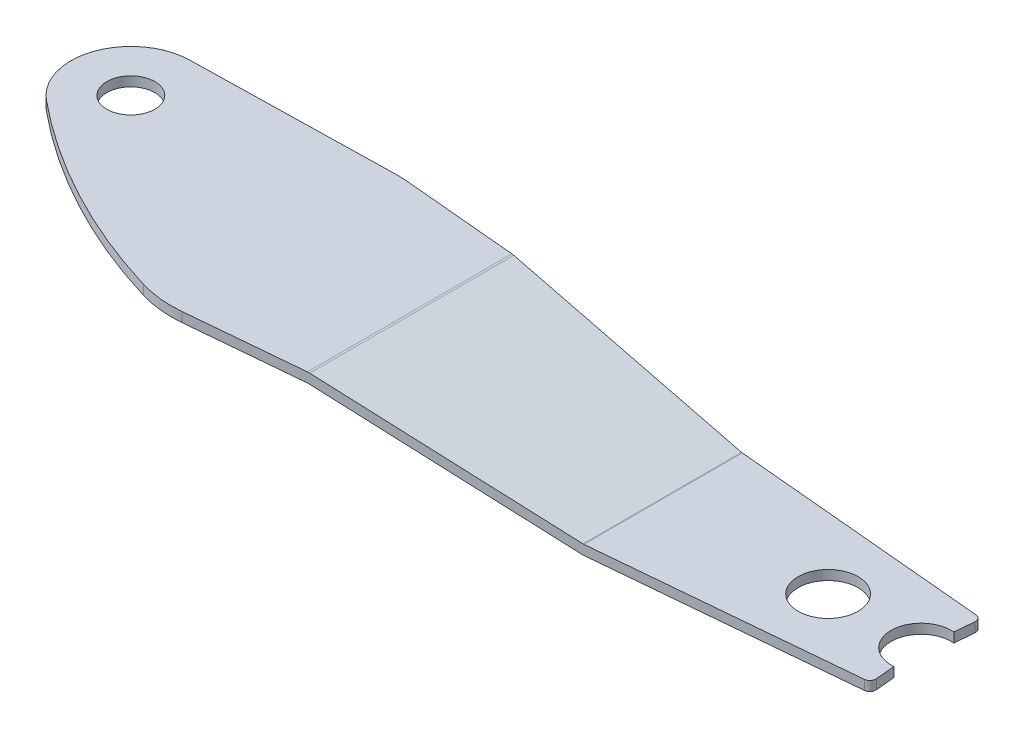
from build123d import *

# Parameters (mm, degrees)
BOSS_EXTRUDE1_DEPTH = 600
SKETCH4_OUTSIDE_W   = 1933.152
SKETCH4_OUTSIDE_H   = 942.352
SKETCH4_OUTSIDE_R   = 40
SKETCH4_OUTSIDE_R_2 = 50
CUT_EXTRUDE1_DEPTH  = 1121.500446229


with BuildPart() as part:
    # Sketch1 → Boss-Extrude1 (new body)
    with BuildSketch(Plane.XY):
        with BuildLine():
            Line((-1.216429586, 8), (-647.3, 8))
            Line((-647.3, 8), (-647.3, -8))
            Line((-647.3, -8), (-1.216429586, -8))
            ThreePointArc((-1.216429586, -8), (-0.542173275, -8.022756973), (0.12901423, -8.090924315))
            Line((0.12901423, -8.090924315), (417.518275664, -64.763596782))
            ThreePointArc((417.518275664, -64.763596782), (419.263363176, -64.940831871), (421.016429586, -65))
            Line((421.016429586, -65), (943.5, -65))
            Line((943.5, -65), (943.5, -49))
            Line((943.5, -49), (421.016429586, -49))
            ThreePointArc((421.016429586, -49), (420.342173275, -48.977243027), (419.67098577, -48.909075685))
            Line((419.67098577, -48.909075685), (2.281724336, 7.763596782))
            ThreePointArc((2.281724336, 7.763596782), (0.536636824, 7.940831871), (-1.216429586, 8))
        make_face()
    extrude(amount=BOSS_EXTRUDE1_DEPTH)

    # Sketch4 outside → Cut-Extrude1 (cut, through all)
    # profile 1 of 3: a face of its own
    with BuildSketch(Plane(origin=(0, 8, 0), x_dir=(1, 0, 0), z_dir=(0, 1, 0))):
        with Locations((148.1, -300)):
            Rectangle(SKETCH4_OUTSIDE_W, SKETCH4_OUTSIDE_H)
        with BuildLine():
            Line((849.441033389, -393.022786976), (-192.741176471, -487.726520609))
            ThreePointArc((-192.741176471, -487.726520609), (-228.733049722, -487.54676651), (-264.034655196, -480.529366519))
            ThreePointArc((-264.034655196, -480.529366519), (-446.549262984, -405.356942265), (-610.742483166, -295.798456192))
            ThreePointArc((-610.742483166, -295.798456192), (-641.798915546, -185.789833988), (-549.379294824, -118.521619672))
            Line((-549.379294824, -118.521619672), (-213.719470744, -111.540753082))
            ThreePointArc((-213.719470744, -111.540753082), (-203.220116273, -111.614875507), (-192.741176471, -112.273479391))
            Line((-192.741176471, -112.273479391), (849.441033389, -206.977213024))
            ThreePointArc((849.441033389, -206.977213024), (856.218024477, -210.53404245), (858.495022624, -217.84115701))
            Line((858.495022624, -217.84115701), (855.553845389, -250.207806915))
            ThreePointArc((855.553845389, -250.207806915), (801, -300), (855.553845389, -349.792193085))
            Line((855.553845389, -349.792193085), (858.495022624, -382.15884299))
            ThreePointArc((858.495022624, -382.15884299), (856.218024477, -389.46595755), (849.441033389, -393.022786976))
        make_face(mode=Mode.SUBTRACT)
    # profile 2 of 3: a face of its own
    with BuildSketch(Plane(origin=(0, 8, 0), x_dir=(1, 0, 0), z_dir=(0, 1, 0))):
        with Locations(Location((-547.3, -218.5, 0), (0, 0, 180))):
            Circle(SKETCH4_OUTSIDE_R)
    # profile 3 of 3: a face of its own
    with BuildSketch(Plane(origin=(0, 8, 0), x_dir=(1, 0, 0), z_dir=(0, 1, 0))):
        with Locations(Location((696, -300, 0), (0, 0, 180))):
            Circle(SKETCH4_OUTSIDE_R_2)
    extrude(amount=-CUT_EXTRUDE1_DEPTH, mode=Mode.SUBTRACT)


solid = part.part
